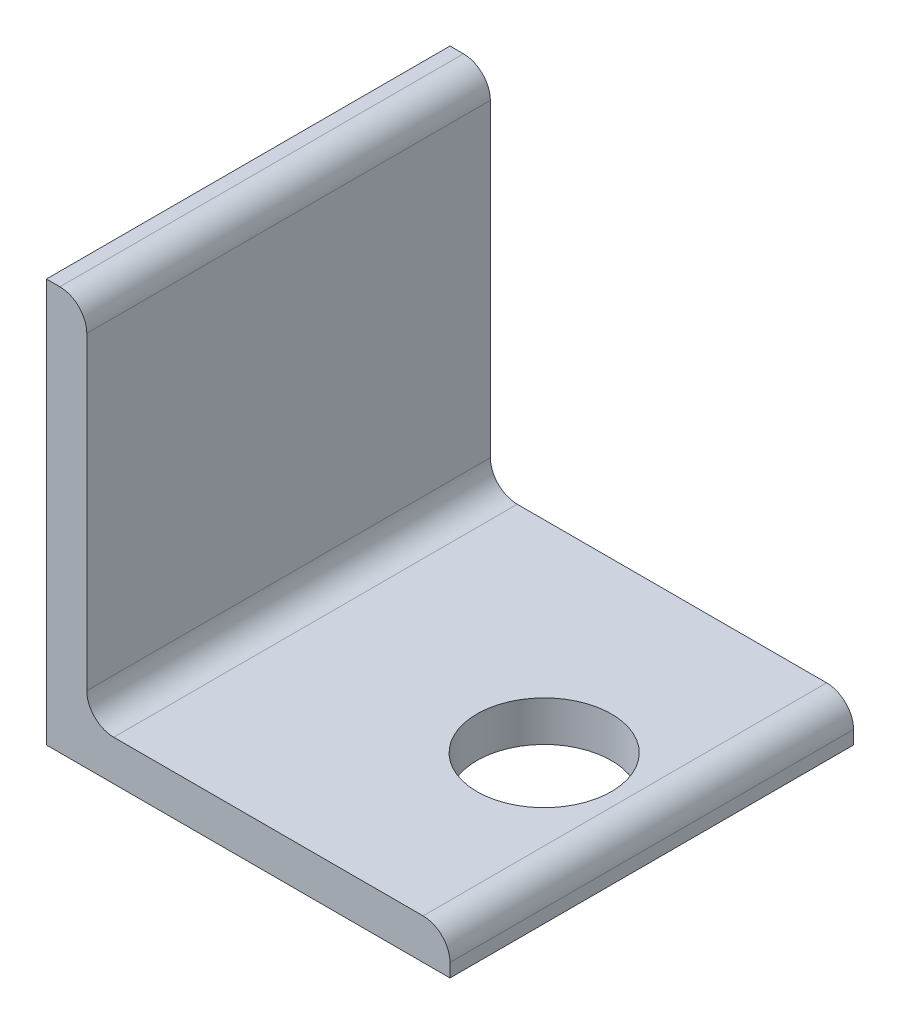
SolidWorks part; units mm, degrees
material "Plain Carbon Steel"
ref_plane "Front Plane" through (0, 0, 0) normal (0, 0, 1) x (1, 0, 0)
ref_plane "Top Plane" through (0, 0, 0) normal (0, 1, 0) x (1, 0, 0)
ref_plane "Right Plane" through (0, 0, 0) normal (1, 0, 0) x (0, 0, -1)
sketch "Sketch2" plane through (0, 0, 0) normal (0, 0, 1) x (1, 0, 0)
  line L0 (0, 0) -> (0, 30)
  line L1 (0, 0) -> (30, 0)
  line L2 (5, 3) -> (28, 3)
  line L3 (3, 5) -> (3, 28)
  line L4 (0, 30) -> (1, 30)
  line L5 (30, 1) -> (30, 0)
  line L6 (3, 3) -> (3, 30) construction
  line L7 (3, 3) -> (30, 3) construction
  arc A0 (3, 28) -> (1, 30) centre (1, 28) ccw
  arc A1 (5, 3) -> (3, 5) centre (5, 5) cw
  arc A2 (30, 1) -> (28, 3) centre (28, 1) ccw
  dimension "D4" = 2
  dimension "D5" = 2
  dimension "D1" = 30
  dimension "D2" = 30
  dimension "D3" = 3
extrude "Boss-Extrude1" add sketch "Sketch2" along normal blind 30
sketch "Sketch3" plane through (0, 3, 0) normal (0, 1, 0) x (1, 0, 0)
  line L0 (0, -30) -> (0, 0) construction
  line L1 (28, 0) -> (5, 0) construction
  circle A0 centre (22, -15) radius 5
  dimension "D1" = 10
  dimension "D2" = 22
  dimension "D3" = 15
extrude "Cut-Extrude1" cut sketch "Sketch3" against normal blind 3
